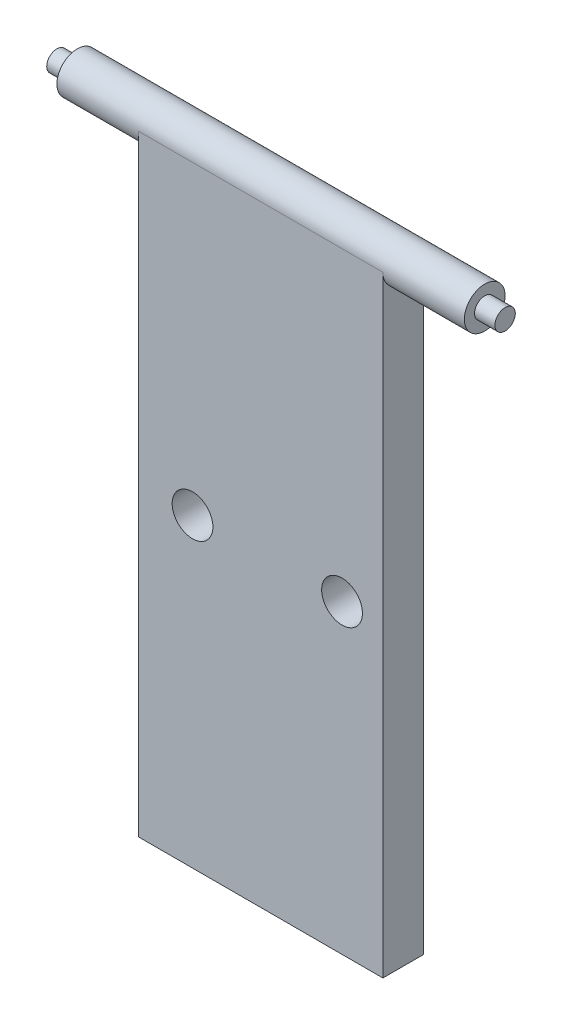
from build123d import *

# Parameters (mm, degrees)
SKETCH1_W                = 60
SKETCH1_H                = 150
BOSS_EXTRUDE1_DEPTH      = 10
SKETCH2_R                = 5
CUT_EXTRUDE1_DEPTH       = 10
BOSS_EXTRUDE2_DEPTH      = 20
BOSS_EXTRUDE2_DEPTH_BACK = 80.0001
SKETCH3_R                = 5
BOSS_EXTRUDE3_DEPTH      = 5
BOSS_EXTRUDE3_DEPTH_BACK = 105
SKETCH4_R                = 2.5


with BuildPart() as part:
    # Sketch1 → Boss-Extrude1 (new body)
    with BuildSketch(Plane.XY):
        Rectangle(SKETCH1_W, SKETCH1_H)
    extrude(amount=BOSS_EXTRUDE1_DEPTH)

    # Sketch2 → Cut-Extrude1 (cut)
    with BuildSketch(Plane.XY.offset(10)):
        with Locations((-16.71752283, 0)):
            Circle(SKETCH2_R)
        with Locations((19.976362571, 0)):
            Circle(SKETCH2_R)
    extrude(amount=-CUT_EXTRUDE1_DEPTH, mode=Mode.SUBTRACT)

    # Sketch3 → Boss-Extrude2 (add, two sides: drawn at the far end of the back side and taken through both)
    with BuildSketch(Plane(origin=(30, 0, 0), x_dir=(0, 0, -1), z_dir=(1, 0, 0)).offset(-BOSS_EXTRUDE2_DEPTH_BACK)):
        with Locations((-5, 75)):
            Circle(SKETCH3_R)
    extrude(amount=BOSS_EXTRUDE2_DEPTH + BOSS_EXTRUDE2_DEPTH_BACK)

    # Sketch4 → Boss-Extrude3 (add, two sides: drawn at the far end of the back side and taken through both)
    with BuildSketch(Plane.ZY.offset(50.0001).offset(-BOSS_EXTRUDE3_DEPTH_BACK)):
        with Locations((5, 75)):
            Circle(SKETCH4_R)
    extrude(amount=BOSS_EXTRUDE3_DEPTH + BOSS_EXTRUDE3_DEPTH_BACK)


solid = part.part
